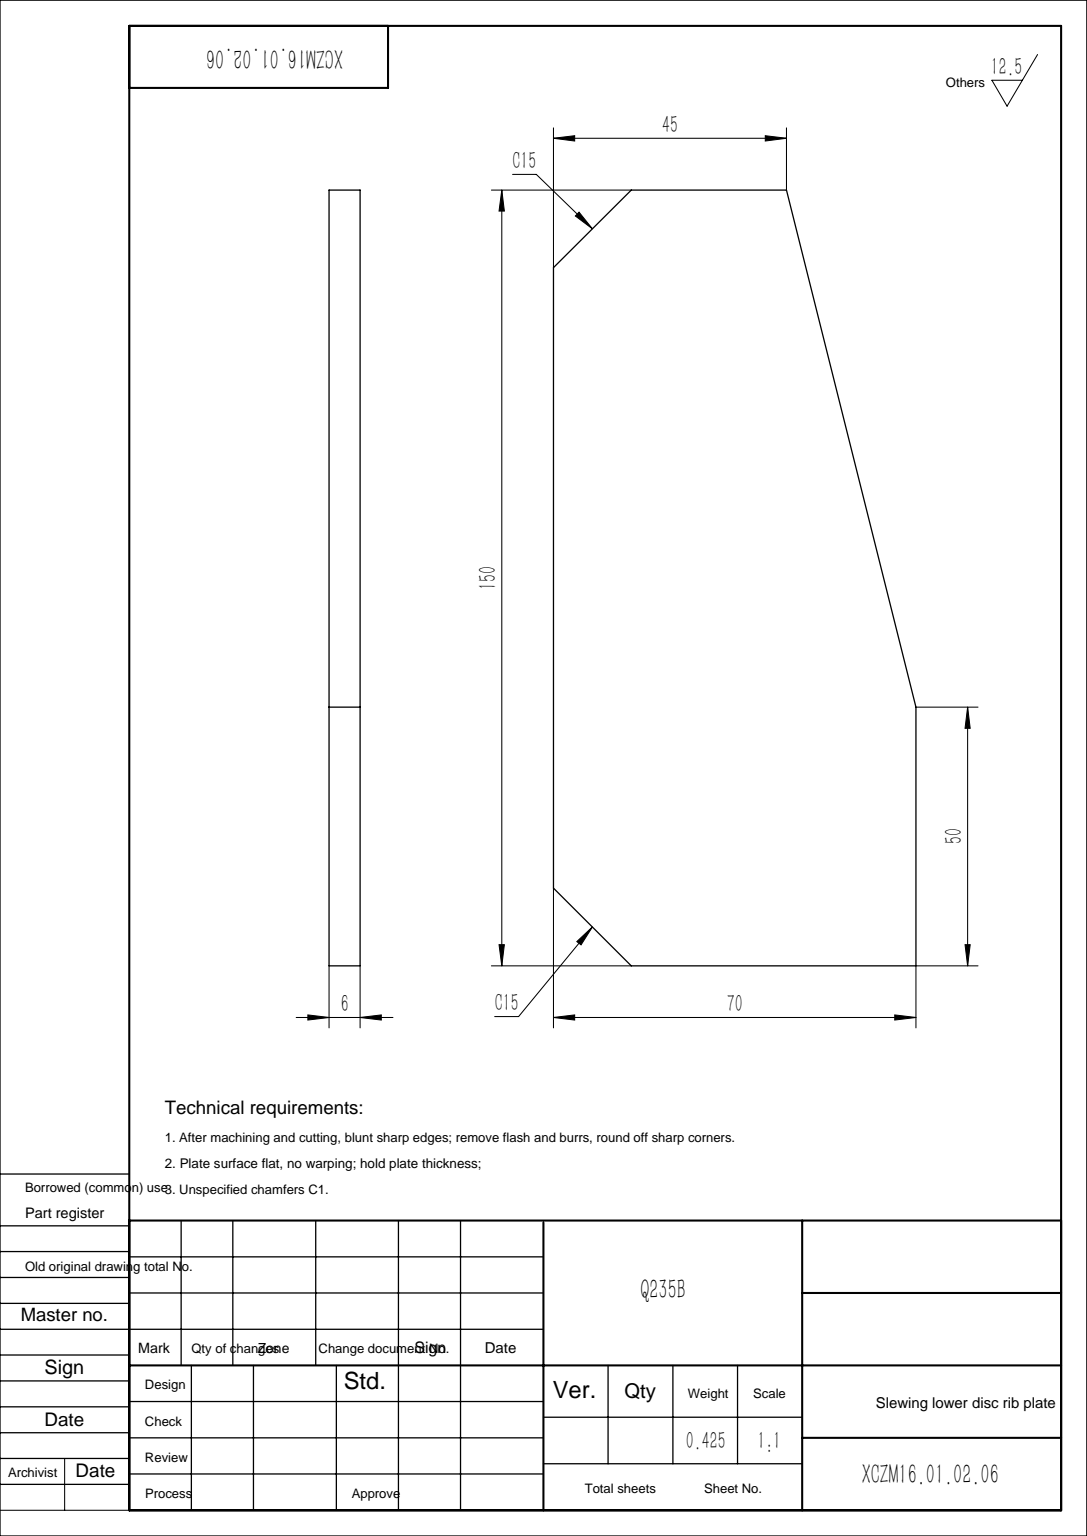
SolidWorks part; units mm, degrees
material "Q235B"
ref_plane "Front Plane" through (0, 0, 0) normal (0, 0, 1) x (1, 0, 0)
ref_plane "Top Plane" through (0, 0, 0) normal (0, 1, 0) x (1, 0, 0)
ref_plane "Right Plane" through (0, 0, 0) normal (1, 0, 0) x (0, 0, -1)
sketch "Sketch1" plane through (0, 0, 0) normal (0, 0, 1) x (1, 0, 0)
  line L0 (0, 150) -> (0, 0)
  line L1 (0, 0) -> (70, 0)
  line L2 (70, 0) -> (70, 50)
  line L3 (70, 50) -> (45, 150)
  line L4 (45, 150) -> (0, 150)
  dimension "D1" = 70
  dimension "D2" = 50
  dimension "D3" = 150
  dimension "D4" = 45
extrude "Boss-Extrude1" add sketch "Sketch1" along normal blind 6
chamfer "Chamfer1" distance 15 angle 45 2 edges at (0, 0, 3) (0, 150, 3)
